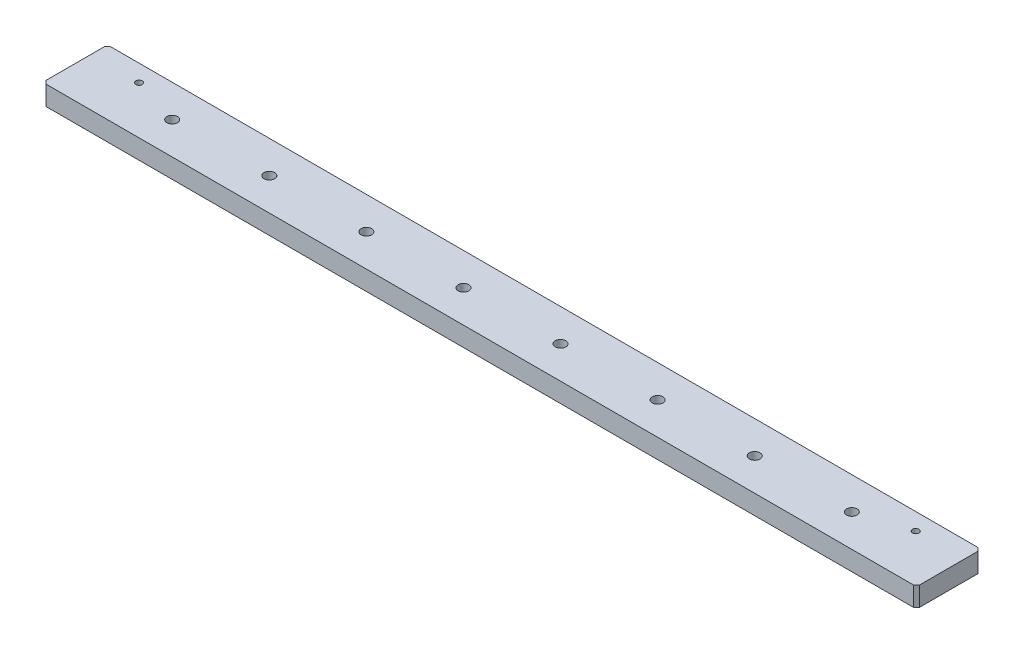
SolidWorks part; units mm, degrees
ref_plane "前视基准面" through (0, 0, 0) normal (0, 0, 1) x (1, 0, 0)
ref_plane "上视基准面" through (0, 0, 0) normal (0, 1, 0) x (1, 0, 0)
ref_plane "右视基准面" through (0, 0, 0) normal (1, 0, 0) x (0, 0, -1)
sketch "草图1" plane through (0, 0, 0) normal (0, 1, 0) x (1, 0, 0)
  line L1 (-270, -20) -> (270, -20)
  line L2 (-270, -20) -> (-270, 20)
  line L3 (-270, 20) -> (270, 20)
  line L4 (270, -20) -> (270, 20)
  line L5 (-270, -20) -> (270, 20) construction
  line L6 (-270, 20) -> (270, -20) construction
  point P0 (0, 0)
  dimension "D1" = 40
  dimension "D2" = 540
extrude "凸台-拉伸1" add sketch "草图1" along normal blind 12
chamfer "倒角1" distance 2 angle 45 4 edges at (270, 6, 20) (-270, 6, 20) (-270, 6, -20) (270, 6, -20)
sketch "草图4" plane through (0, 0, 0) normal (0, -1, 0) x (-1, 0, 0)
  line L0 (-268, 20) -> (268, 20) construction
  line L1 (-270, -18) -> (-270, 18) construction
  line L2 (0, -20) -> (0, 87.1137) construction
  line L3 (268, -20) -> (-268, -20) construction
  point P0 (-240, 9.5)
  point P14 (240, 9.5)
  dimension "D1" = 10.5
  dimension "D2" = 30
hole_wizard "Ø4.0mm 暗销孔1" positions "草图4" profile "草图3" hole size "Ø4.0" standard "GB"
sketch "草图3" plane through (240, 0, -9.5) normal (1, 0, 0) x (0, 0, -1)
  line L0 (0, 0) -> (0, 13.2017)
  line L1 (0, 13.2017) -> (2, 12)
  line L2 (2, 12) -> (2, 0)
  line L5 (2, 0) -> (0, 0)
  line L10 (0, 13.2017) -> (-2, 12) construction
  line L11 (0, -6.35) -> (0, 107.95) construction
  dimension "孔直径" = 4
  dimension "孔深度" = 12
  dimension "导头角度" = 118
sketch "草图7" plane through (0, 0, 0) normal (0, -1, 0) x (-1, 0, 0)
  point P0 (-240, 0)
hole_wizard "M3 螺纹孔1" positions "草图7" profile "草图6" tap size "M3" standard "GB"
sketch "草图6" plane through (240, 0, 0) normal (1, 0, 0) x (0, 0, -1)
  line L0 (0, 0) -> (0, 8.2511)
  line L1 (0, 8.2511) -> (1.25, 7.5)
  line L2 (1.25, 7.5) -> (1.25, 0)
  line L5 (1.25, 0) -> (0, 0)
  line L10 (0, 8.2511) -> (-1.25, 7.5) construction
  line L11 (0, -6.35) -> (0, 107.95) construction
  dimension "螺纹孔钻头直径" = 2.5
  dimension "螺纹孔钻头深度" = 7.5
  dimension "导头角度" = 118
cosmetic thread "孔螺纹线1" parameters "D1"=6, "D2"=3
pattern_linear "阵列(线性)4" count 9 spacing 60 along (-1, 0, 0) of "M3 螺纹孔1"
sketch "草图10" plane through (0, 0, 0) normal (0, -1, 0) x (-1, 0, 0)
  line L0 (270, 18) -> (270, -18) construction
  point P0 (210, 0)
  point P7 (270, 0)
  dimension "D1" = 30
hole_wizard "M6 六角圆柱头螺钉的柱形沉头孔1" positions "草图10" profile "草图9" counterbore size "M6" standard "GB" end condition through all
sketch "草图9" plane through (-210, 0, 0) normal (1, 0, 0) x (0, 0, -1)
  line L0 (0, 0) -> (0, 12)
  line L1 (0, 12) -> (3.3, 12)
  line L3 (3.3, 12) -> (3.3, 6.8)
  line L4 (3.3, 6.8) -> (5.5, 6.8)
  line L5 (5.5, 6.8) -> (5.5, 0)
  line L7 (5.5, 0) -> (0, 0)
  line L11 (0, -6.35) -> (0, 107.95) construction
  dimension "通孔孔直径" = 6.6
  dimension "通孔孔深度" = 12
  dimension "柱形沉头孔直径" = 11
  dimension "柱形沉头孔深度" = 6.8
pattern_linear "阵列(线性)5" count 8 spacing 60 along (1, 0, 0) of "M6 六角圆柱头螺钉的柱形沉头孔1"
